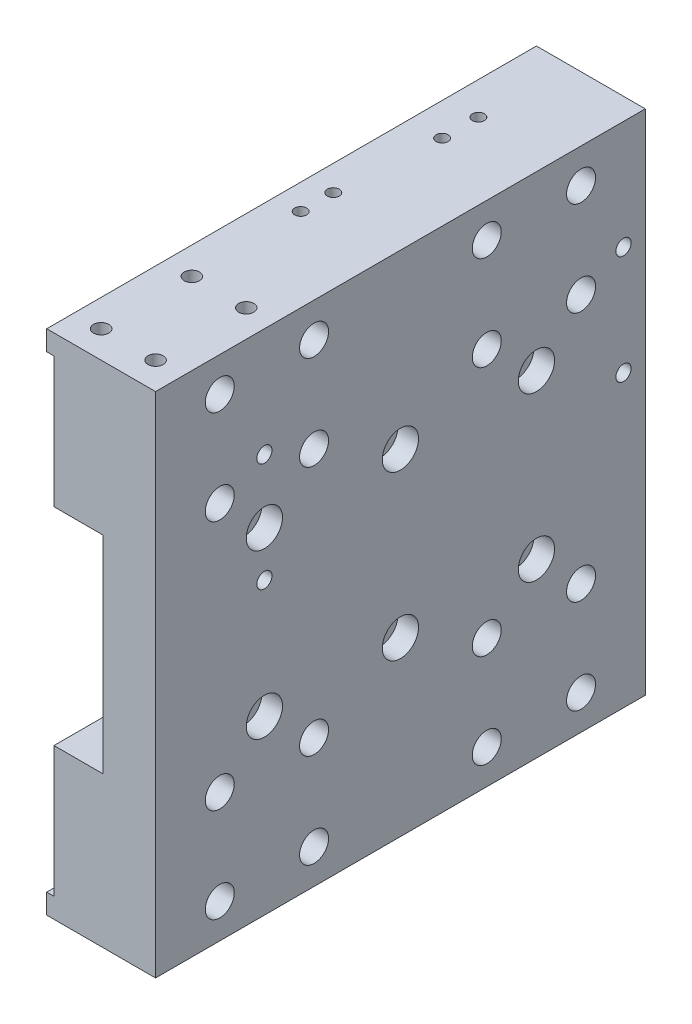
SolidWorks part; units mm, degrees
material "AL6061"
ref_plane "Front Plane" through (0, 0, 0) normal (0, 0, 1) x (1, 0, 0)
ref_plane "Top Plane" through (0, 0, 0) normal (0, 1, 0) x (1, 0, 0)
ref_plane "Right Plane" through (0, 0, 0) normal (1, 0, 0) x (0, 0, -1)
sketch "Sketch1" plane through (0, 0, 0) normal (1, 0, 0) x (0, 0, -1)
  line L1 (-67.5, -70) -> (67.5, -70)
  line L2 (-67.5, -70) -> (-67.5, 70)
  line L3 (-67.5, 70) -> (67.5, 70)
  line L4 (67.5, -70) -> (67.5, 70)
  line L5 (-67.5, -70) -> (67.5, 70) construction
  line L6 (-67.5, 70) -> (67.5, -70) construction
  point P0 (0, 0)
  dimension "D1" = 140
  dimension "D2" = 135
extrude "Boss-Extrude1" add sketch "Sketch1" along normal blind 30
sketch "Sketch2" plane through (0, 0, -67.5) normal (0, 0, -1) x (-1, 0, 0)
  line L0 (0, 0) -> (-30, 0) construction
  line L2 (0, -70) -> (0, 70) construction
  line L3 (-15.5, -28.5) -> (0, -28.5)
  line L4 (-15.5, -28.5) -> (-15.5, 28.5)
  line L5 (-15.5, 28.5) -> (0, 28.5)
  line L6 (0, -28.5) -> (0, 28.5)
  line L7 (-15.5, -28.5) -> (0, 28.5) construction
  line L8 (-15.5, 28.5) -> (0, -28.5) construction
  line L10 (-30, -70) -> (-30, 70) construction
  point P5 (-7.75, 0)
  dimension "D1" = 15.5
  dimension "D2" = 57
extrude "Cut-Extrude1" cut sketch "Sketch2" against normal through all
sketch "Sketch3" plane through (0, 0, 0) normal (-1, 0, 0) x (0, 0, 1)
  line L1 (0, 0) -> (-67.5, 0) construction
  line L2 (67.5, 70) -> (67.5, 28.5) construction
  line L3 (-67.5, -64.5) -> (67.5, -64.5)
  line L4 (-67.5, -64.5) -> (-67.5, 64.5)
  line L5 (-67.5, 64.5) -> (67.5, 64.5)
  line L6 (67.5, -64.5) -> (67.5, 64.5)
  line L7 (-67.5, -64.5) -> (67.5, 64.5) construction
  line L8 (-67.5, 64.5) -> (67.5, -64.5) construction
  line L9 (-67.5, -70) -> (-67.5, -28.5) construction
  line L10 (-67.5, 28.5) -> (-67.5, -28.5) construction
  dimension "D1" = 129
extrude "Cut-Extrude2" cut sketch "Sketch3" against normal blind 2
hole_wizard "M4 Tapped Hole1" positions "Sketch4" profile "Sketch5" tap size "M4" standard "GB"
sketch "Sketch4" plane through (0, 70, 0) normal (0, 1, 0) x (1, 0, 0)
  point P0 (7, 4.5)
  point P3 (7, -4.5)
sketch "Sketch5" plane through (7, 70, -4.5) normal (1, 0, 0) x (0, 0, 1)
  line L0 (0, 0) -> (0, 11.0914)
  line L1 (0, 11.0914) -> (1.65, 10.1)
  line L2 (1.65, 10.1) -> (1.65, 0)
  line L5 (1.65, 0) -> (0, 0)
  line L10 (0, 11.0914) -> (-1.65, 10.1) construction
  line L11 (0, -6.35) -> (0, 107.95) construction
  dimension "螺纹孔钻头直径" = 3.3
  dimension "螺纹孔钻头深度" = 10.1
  dimension "导头角度" = 118
cosmetic thread "Cosmetic thread1" parameters "D1"=8, "D2"=4
cosmetic thread "Cosmetic thread2" parameters "D1"=8, "D2"=4
hole_wizard "M5 Tapped Hole1" positions "Sketch6" profile "Sketch7" tap size "M5" standard "GB"
sketch "Sketch6" plane through (0, -70, 0) normal (0, -1, 0) x (-1, 0, 0)
  line L1 (-15, 67.5) -> (-15, -67.5) construction
  line L2 (-30, 67.5) -> (0, 67.5) construction
  line L3 (-30, -67.5) -> (0, -67.5) construction
  line L5 (0, 0) -> (-30, 0) construction
  line L6 (-30, -67.5) -> (-30, 67.5) construction
  point P0 (-24, 33.75)
  point P3 (-6, 33.75)
  point P6 (-24, -33.75)
  point P9 (-6, -33.75)
  dimension "D1" = 67.5
  dimension "D2" = 18
sketch "Sketch7" plane through (24, -70, -33.75) normal (1, 0, 0) x (0, 0, -1)
  line L0 (0, 0) -> (0, 13.6618)
  line L1 (0, 13.6618) -> (2.1, 12.4)
  line L2 (2.1, 12.4) -> (2.1, 0)
  line L5 (2.1, 0) -> (0, 0)
  line L10 (0, 13.6618) -> (-2.1, 12.4) construction
  line L11 (0, -6.35) -> (0, 107.95) construction
  dimension "螺纹孔钻头直径" = 4.2
  dimension "螺纹孔钻头深度" = 12.4
  dimension "导头角度" = 118
cosmetic thread "Cosmetic thread25" parameters "D1"=10, "D2"=5.2
cosmetic thread "Cosmetic thread26" parameters "D1"=10, "D2"=5.2
cosmetic thread "Cosmetic thread27" parameters "D1"=10, "D2"=5.2
cosmetic thread "Cosmetic thread28" parameters "D1"=10, "D2"=5.2
hole_wizard "Ø5.0mm dowel hole1" positions "Sketch8" profile "Sketch9" hole size "Ø5.0" standard "GB"
sketch "Sketch8" plane through (0, -70, 0) normal (0, -1, 0) x (-1, 0, 0)
  line L0 (-24, 33.75) -> (-6, 33.75) construction
  line L2 (-24, -33.75) -> (-6, -33.75) construction
  point P0 (-15, 33.75)
  point P3 (-15, -33.75)
sketch "Sketch9" plane through (15, -70, -33.75) normal (1, 0, 0) x (0, 0, -1)
  line L0 (0, 0) -> (0, 9.5022)
  line L1 (0, 9.5022) -> (2.5, 8)
  line L2 (2.5, 8) -> (2.5, 0)
  line L5 (2.5, 0) -> (0, 0)
  line L10 (0, 9.5022) -> (-2.5, 8) construction
  line L11 (0, -6.35) -> (0, 107.95) construction
  dimension "孔直径" = 5
  dimension "孔深度" = 8
  dimension "导头角度" = 118
hole_wizard "M5 Tapped Hole2" positions "Sketch10" profile "Sketch11" tap size "M5" standard "GB"
sketch "Sketch10" plane through (30, 0, 0) normal (1, 0, 0) x (0, 0, -1)
  point P0 (-37.5, 40)
  point P3 (-37.5, 10)
  point P6 (61.5, 40)
  point P9 (61.5, 10)
sketch "Sketch11" plane through (30, 40, 37.5) normal (0, 1, 0) x (0, 0, -1)
  line L0 (0, 0) -> (0, 13.6618)
  line L1 (0, 13.6618) -> (2.1, 12.4)
  line L2 (2.1, 12.4) -> (2.1, 0)
  line L5 (2.1, 0) -> (0, 0)
  line L10 (0, 13.6618) -> (-2.1, 12.4) construction
  line L11 (0, -6.35) -> (0, 107.95) construction
  dimension "螺纹孔钻头直径" = 4.2
  dimension "螺纹孔钻头深度" = 12.4
  dimension "导头角度" = 118
cosmetic thread "Cosmetic thread7" parameters "D1"=10, "D2"=5
cosmetic thread "Cosmetic thread8" parameters "D1"=10, "D2"=5
cosmetic thread "Cosmetic thread9" parameters "D1"=10, "D2"=5
cosmetic thread "Cosmetic thread10" parameters "D1"=10, "D2"=5
hole_wizard "CBORE for M4 Hexagon socket head cap screws1" positions "Sketch14" profile "Sketch16" counterbore size "M4" standard "GB" end condition through all
sketch "Sketch14" plane through (30, 0, 0) normal (1, 0, 0) x (0, 0, -1)
  line L0 (0, 70) -> (0, -70) construction
  line L1 (67.5, 70) -> (-67.5, 70) construction
  line L2 (-67.5, -70) -> (67.5, -70) construction
  line L4 (67.5, 0) -> (-67.5, 0) construction
  line L5 (67.5, -70) -> (67.5, 70) construction
  line L6 (-67.5, 70) -> (-67.5, -70) construction
  point P0 (-49.8, 60.5)
  point P2 (-23.8, 60.5)
  point P4 (-23.8, 34.5)
  point P6 (-49.8, 34.5)
  point P29 (49.8, 34.5)
  point P30 (23.8, 34.5)
  point P31 (23.8, 60.5)
  point P32 (49.8, 60.5)
  point P33 (49.8, -60.5)
  point P34 (23.8, -60.5)
  point P35 (23.8, -34.5)
  point P36 (49.8, -34.5)
  point P37 (-49.8, -34.5)
  point P38 (-23.8, -34.5)
  point P39 (-23.8, -60.5)
  point P40 (-49.8, -60.5)
  dimension "D1" = 26
  dimension "D2" = 26
  dimension "D3" = 69
  dimension "D4" = 47.6
sketch "Sketch16" plane through (30, 60.5, 49.8) normal (0, 1, 0) x (0, 0, -1)
  line L0 (0, 0) -> (0, 30)
  line L1 (0, 30) -> (2.25, 30)
  line L3 (2.25, 30) -> (2.25, 23)
  line L4 (2.25, 23) -> (4, 23)
  line L5 (4, 23) -> (4, 0)
  line L7 (4, 0) -> (0, 0)
  line L11 (0, -6.35) -> (0, 107.95) construction
  dimension "通孔孔直径" = 4.5
  dimension "通孔孔深度" = 30
  dimension "柱形沉头孔直径" = 8
  dimension "柱形沉头孔深度" = 23
hole_wizard "CBORE for M5 Hexagon socket head cap screws1" positions "Sketch19" profile "Sketch20" counterbore size "M5" standard "GB" end condition through all
sketch "Sketch19" plane through (30, 0, 0) normal (1, 0, 0) x (0, 0, -1)
  line L0 (-67.5, 0) -> (67.5, 0) construction
  line L1 (-67.5, 70) -> (-67.5, -70) construction
  line L2 (67.5, -70) -> (67.5, 70) construction
  line L4 (0, 70) -> (0, -70) construction
  line L5 (67.5, 70) -> (-67.5, 70) construction
  line L6 (-67.5, -70) -> (67.5, -70) construction
  point P0 (0, 22.5)
  point P2 (0, -22.5)
  dimension "D1" = 45
sketch "Sketch20" plane through (30, 22.5, 0) normal (0, 1, 0) x (0, 0, -1)
  line L0 (0, 0) -> (0, 30)
  line L1 (0, 30) -> (2.75, 30)
  line L3 (2.75, 30) -> (2.75, 5.7)
  line L4 (2.75, 5.7) -> (5, 5.7)
  line L5 (5, 5.7) -> (5, 0)
  line L7 (5, 0) -> (0, 0)
  line L11 (0, -6.35) -> (0, 107.95) construction
  dimension "通孔孔直径" = 5.5
  dimension "通孔孔深度" = 30
  dimension "柱形沉头孔直径" = 10
  dimension "柱形沉头孔深度" = 5.7
pattern_linear "LPattern1" count 2 spacing 37.5 along (0, 0, 1) count 2 spacing 37.5 along (0, 0, -1) seed only of "CBORE for M5 Hexagon socket head cap screws1"
hole_wizard "M5 Tapped Hole3" positions "Sketch23" profile "Sketch24" tap size "M5" standard "GB"
sketch "Sketch23" plane through (0, 70, 0) normal (0, 1, 0) x (1, 0, 0)
  line L0 (30, -67.5) -> (0, -67.5) construction
  line L1 (15, -67.5) -> (15, 67.5) construction
  line L2 (30, 67.5) -> (0, 67.5) construction
  point P0 (7.5, -60)
  point P2 (22.5, -60)
  point P4 (22.5, -35)
  point P6 (7.5, -35)
  dimension "D1" = 15
  dimension "D2" = 25
  dimension "D3" = 7.5
sketch "Sketch24" plane through (7.5, 70, 60) normal (1, 0, 0) x (0, 0, 1)
  line L0 (0, 0) -> (0, 13.6618)
  line L1 (0, 13.6618) -> (2.1, 12.4)
  line L2 (2.1, 12.4) -> (2.1, 0)
  line L5 (2.1, 0) -> (0, 0)
  line L10 (0, 13.6618) -> (-2.1, 12.4) construction
  line L11 (0, -6.35) -> (0, 107.95) construction
  dimension "螺纹孔钻头直径" = 4.2
  dimension "螺纹孔钻头深度" = 12.4
  dimension "导头角度" = 118
cosmetic thread "Cosmetic thread11" parameters "D1"=10, "D2"=5
cosmetic thread "Cosmetic thread12" parameters "D1"=10, "D2"=5
cosmetic thread "Cosmetic thread13" parameters "D1"=10, "D2"=5
cosmetic thread "Cosmetic thread14" parameters "D1"=10, "D2"=5
hole_wizard "M4 Tapped Hole2" positions "Sketch27" profile "Sketch28" tap size "M4" standard "GB"
sketch "Sketch27" plane through (0, 70, 0) normal (0, 1, 0) x (1, 0, 0)
  line L0 (30, 67.5) -> (0, 67.5) construction
  line L1 (0, 67.5) -> (0, -67.5) construction
  point P0 (9, 42.5)
  point P2 (9, 32.5)
  dimension "D1" = 25
  dimension "D2" = 10
  dimension "D3" = 9
sketch "Sketch28" plane through (9, 70, -42.5) normal (1, 0, 0) x (0, 0, 1)
  line L0 (0, 0) -> (0, 11.0914)
  line L1 (0, 11.0914) -> (1.65, 10.1)
  line L2 (1.65, 10.1) -> (1.65, 0)
  line L5 (1.65, 0) -> (0, 0)
  line L10 (0, 11.0914) -> (-1.65, 10.1) construction
  line L11 (0, -6.35) -> (0, 107.95) construction
  dimension "螺纹孔钻头直径" = 3.3
  dimension "螺纹孔钻头深度" = 10.1
  dimension "导头角度" = 118
cosmetic thread "Cosmetic thread15" parameters "D1"=8, "D2"=4
cosmetic thread "Cosmetic thread16" parameters "D1"=8, "D2"=4
